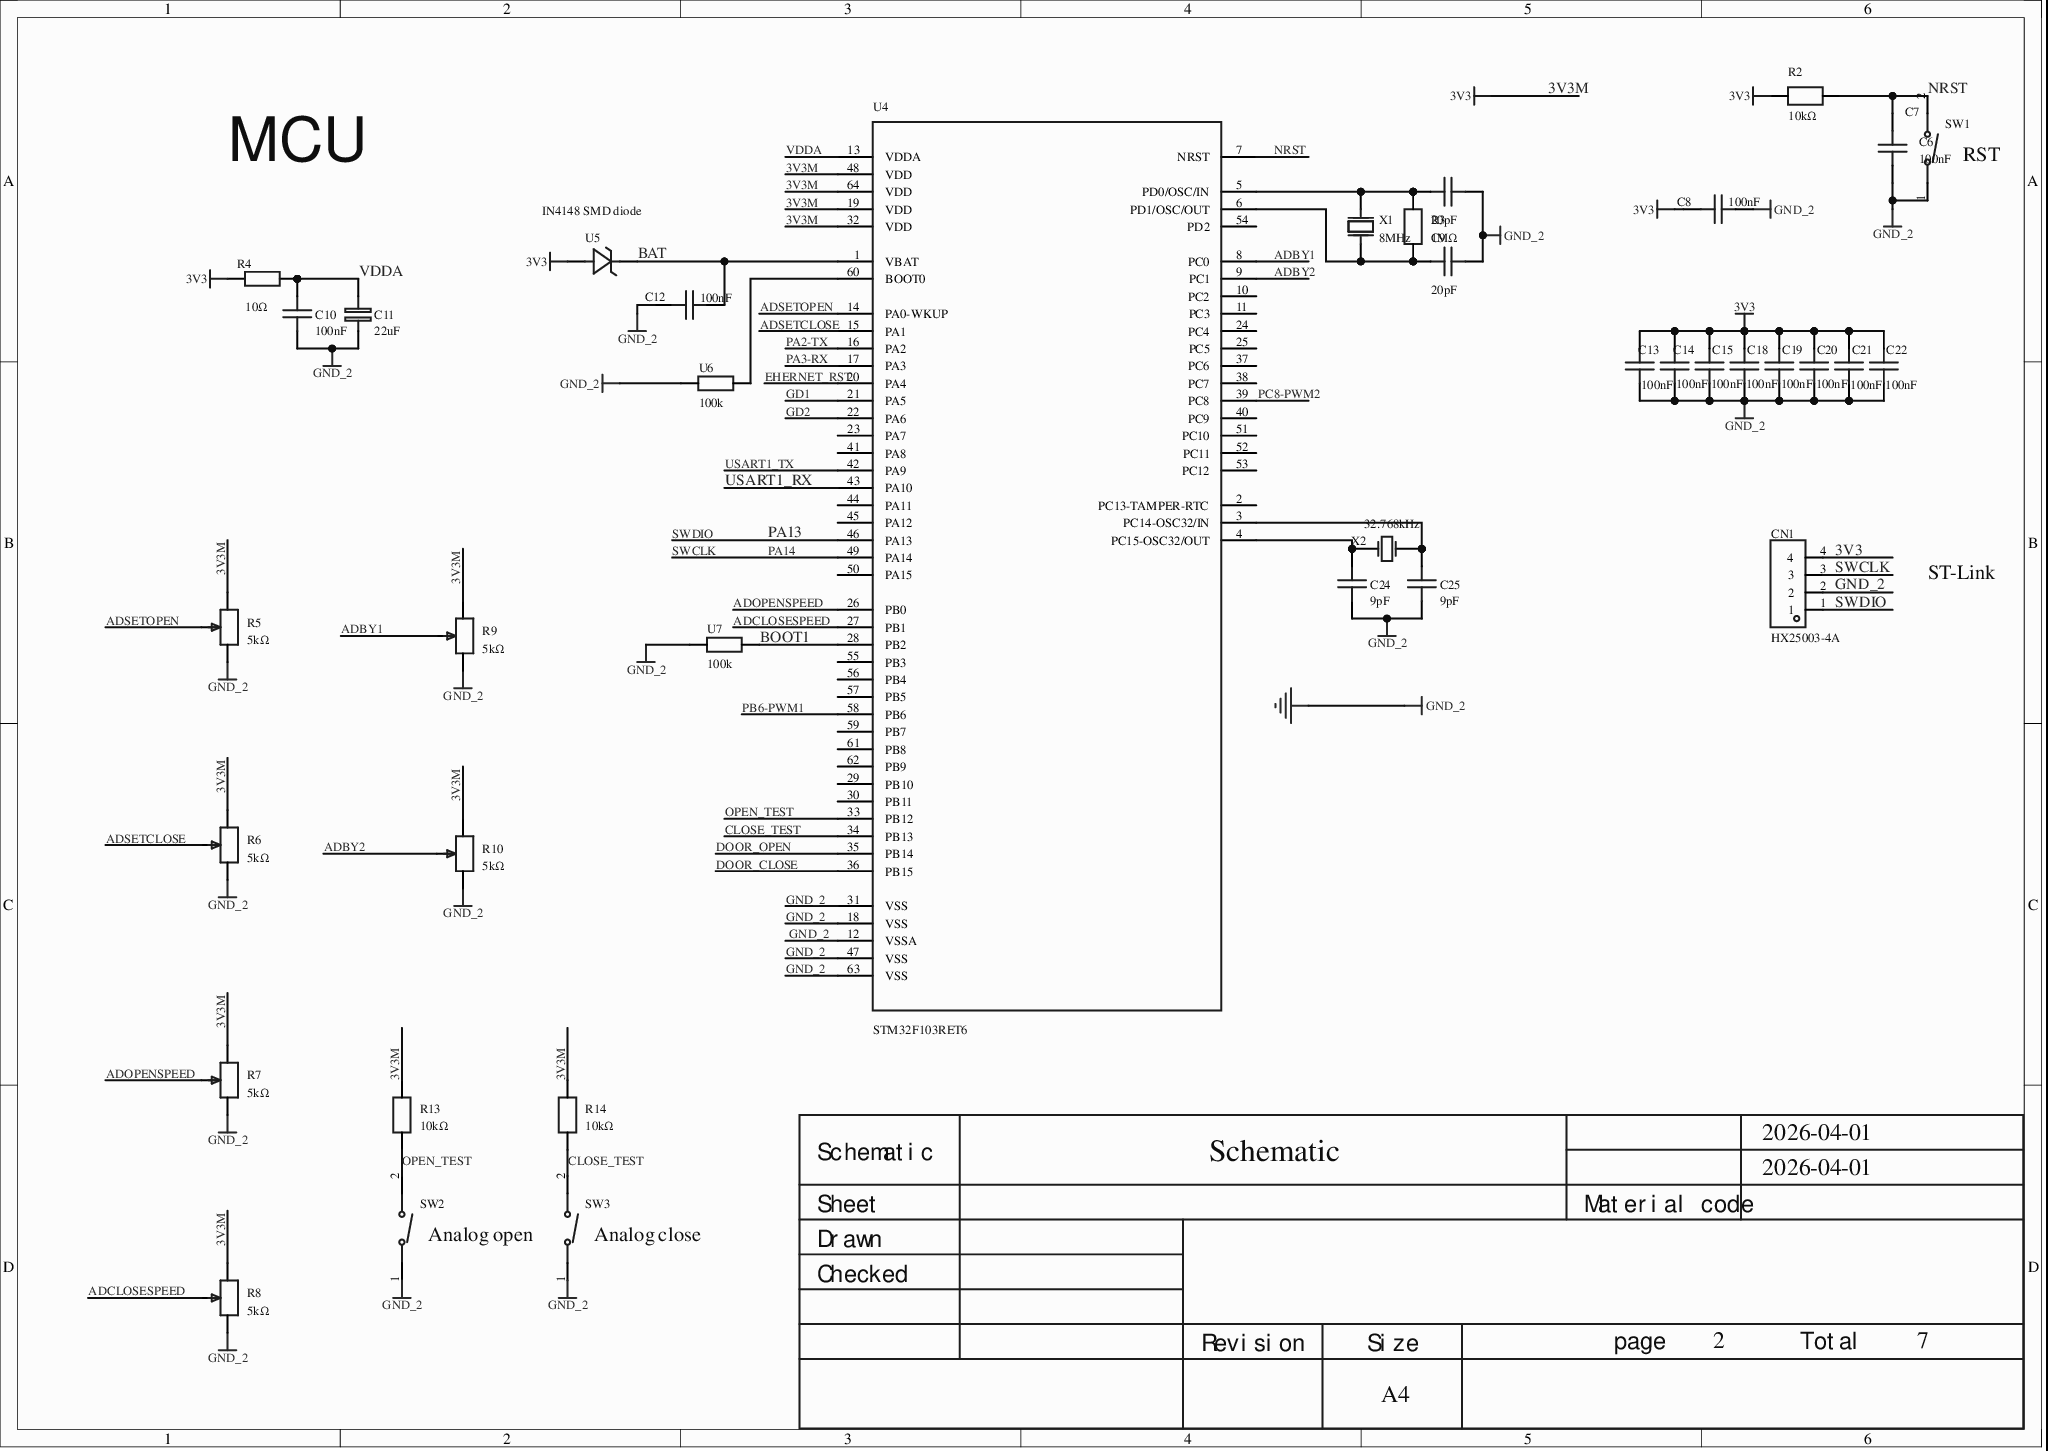
[diagram p0: MISC49876-3.schdoc]
# Altium project MISC49876-2.PrjPcb (part 1 of 2)
3 sheets, 90 parts. Net scope: global (net labels, ports and power ports of the same name join across sheets).
Board file: MISC49876.pcbdoc
Sheets:
  MISC49876-3.schdoc
  MISC49876-5.schdoc
  MISC49876-4.schdoc

## Sheet MISC49876-3.schdoc
size 297 x 210 mm; Version: V1.0; @Project Name: MISC49876; @Page Count: 7; @Update Date: 2026-04-01; @Create Date: 2026-04-01; @Schematic Name: MISC49876; @Page No: 2; @Board Name: MISC49876; @Create Time: 08:05:42; @Update Time: 16:05:42

### Parts
C6  100nF  [C0603]
C7  20pF  [C0603]
C8  100nF  [C0603]
C9  20pF  [C0603]
C10  100nF  [C0603]
C11  22uF  [C0603]
C12  100nF  [C0603]
C13  100nF  [C0603]
C14  100nF  [C0603]
C15  100nF  [C0603]
C18  100nF  [C0603]
C19  100nF  [C0603]
C20  100nF  [C0603]
C21  100nF  [C0603]
C22  100nF  [C0603]
C24  9pF  [C0402]
C25  9pF  [C0402]
CN1  HX25003-4A  [CONN-TH_4P-P2.50_HX25003-4A]
R2  10kΩ  [R0603]
R3  1MΩ  [R0603]
R4  10Ω  [R0603]
R5  5kΩ  [RES-ADJ-TH_3296W-1-203]
R6  5kΩ  [RES-ADJ-TH_3296W-1-203]
R7  5kΩ  [RES-ADJ-TH_3296W-1-203]
R8  5kΩ  [RES-ADJ-TH_3296W-1-203]
R9  5kΩ  [RES-ADJ-TH_3296W-1-203]
R10  5kΩ  [RES-ADJ-TH_3296W-1-203]
R13  10kΩ  [R0603]
R14  10kΩ  [R0603]
SW1  TS-1101-C-W  [SW-SMD_L6.0-W3.3-LS8.0]  (value not drawn)
SW2  TS-1101-C-W  [SW-SMD_L6.0-W3.3-LS8.0]  (value not drawn)
SW3  TS-1101-C-W  [SW-SMD_L6.0-W3.3-LS8.0]  (value not drawn)
U4  STM32F103RET6  [LQFP-64_L10.0-W10.0-P0.50-LS12.0-BL]
U5  IN4148 SMD diode  [SOD-123_L2.7-W1.7-LS3.8-RD]
U6  100k  [R0603]
U7  100k  [R0603]
X1  8MHz  [CRYSTAL-SMD_L11.5-W4.8-LS12.7]
X2  32.768kHz  [OSC-SMD_L3.2-W1.5]

### Nets
3V3: C8.1 C13.2 C14.2 C15.2 C18.2 C19.2 C20.2 C21.2 C22.2 CN1.4 R2.1 R4.1 R5.3 R6.3 R7.3 R8.3 R9.3 R10.3 R13.1 R14.1 U4.19(VDD) U4.32(VDD) U4.48(VDD) U4.64(VDD) U5.2(A)  [also labelled 3V3M]
GND_2: C6.2 C7.1 C8.2 C9.1 C10.1 C11.1 C12.1 C13.1 C14.1 C15.1 C18.1 C19.1 C20.1 C21.1 C22.1 C24.1 C25.1 CN1.2 R5.1 R6.1 R7.1 R8.1 R9.1 R10.1 SW1.1(A) SW2.1(A) SW3.1(A) U4.12(VSSA) U4.18(VSS) U4.31(VSS) U4.47(VSS) U4.63(VSS) U6.2 U7.1  [also labelled GND]
ADBY1: R9.2 U4.8(PC0)
ADBY2: R10.2 U4.9(PC1)
ADCLOSESPEED: R8.2 U4.27(PB1)
ADOPENSPEED: R7.2 U4.26(PB0)
ADSETCLOSE: R6.2 U4.15(PA1)
ADSETOPEN: R5.2 U4.14(PA0-WKUP)
BAT: C12.2 U4.1(VBAT) U5.1(K)
BOOT1: U4.28(PB2) U7.2
CLOSE_TEST: R14.2 SW3.2(B) U4.34(PB13)
DOOR_CLOSE: U4.36(PB15)
DOOR_OPEN: U4.35(PB14)
EHERNET_RST: U4.20(PA4)
GD1: U4.21(PA5)
GD2: U4.22(PA6)
NRST: C6.1 R2.2 SW1.2(B) U4.7(NRST)
OPEN_TEST: R13.2 SW2.2(B) U4.33(PB12)
PA2-TX: U4.16(PA2)
PA3-RX: U4.17(PA3)
PA13: CN1.1 U4.46(PA13)  [also labelled SWDIO]
PA14: CN1.3 U4.49(PA14)  [also labelled SWCLK]
PB6-PWM1: U4.58(PB6)
PC8-PWM2: U4.39(PC8)
USART1_RX: U4.43(PA10)
USART1_TX: U4.42(PA9)
VDDA: C10.2 C11.2 R4.2 U4.13(VDDA)
NetC7_2: C7.2 R3.1 U4.5(PD0/OSC/IN) X1.1(OSC1)
NetC9_2: C9.2 R3.2 U4.6(PD1/OSC/OUT) X1.2(OSC2)
NetC24_2: C24.2 U4.4(PC15-OSC32/OUT) X2.2(OSC2)
NetC25_2: C25.2 U4.3(PC14-OSC32/IN) X2.1(OSC1)
NetU4_60: U4.60(BOOT0) U6.1

Not connected (* = marked no-connect by the designer): U4 2(PC13-TAMPER-RTC) 10(PC2) 11(PC3) 23(PA7) 24(PC4) 25(PC5) 29(PB10) 30(PB11) 37(PC6) 38(PC7) 40(PC9) 41(PA8) 44(PA11) 45(PA12) 50(PA15) 51(PC10) 52(PC11) 53(PC12) 54(PD2) 55(PB3) 56(PB4) 57(PB5) 59(PB7) 61(PB8) 62(PB9)

### Notes on the sheet
- MCU
- (near SW1) RST
- ST-Link
- Analog open
- (near SW3) Analog close
- 2026-04-01
- Schematic
- Sheet
- Material code
- Checked
- Drawn
- Revision
- Size
- A4
- page
- 2
- Total
- 7

### Library data of the parts
C6 C8 C12-C15 C18-C22 = CC0603KRX7R9BB104: Capacitance: 100nF; tolerance: ±10%; rated voltage: 50V; dielectric (temp. coefficient): X7R;; Manufacturer: YAGEO(国巨); Symbol: 0.1u; Convert to PCB: yes; ModelId: ac125912035d415993ca9572d50418b1; ModelName: C0603_L1.6-W0.8-H0.8; ModelTransform: 62.992,31.496,0,0,0,0,0,0,0; Origin Footprint: C0603; Device: CC0603KRX7R9BB104; Supplier Part: C14663; Supplier: LCSC; Manufacturer Part: CC0603KRX7R9BB104; Add into BOM: yes; JLCPCB Part Class: Basic Part; LCSC Part Name: 100nF ±10% 50V; Supplier Footprint: 0603; Datasheet: https://atta.szlcsc.com/upload/public/pdf/source/20180910/C282072_33301C7F631E79921B82A8DAC6BCC5B3.pdf; FootprintName: C0603; Value: 100nF; Tolerance: ±10%; Voltage Rated: 50V; Temperature Coefficient: X7R
C7 C9 = CC0603JRNPO9BN200: Capacitance: 20pF; tolerance: ±5%; rated voltage: 50V; dielectric (temp. coefficient): NP0;; Manufacturer: YAGEO(国巨); Convert to PCB: yes; ModelId: ac125912035d415993ca9572d50418b1; ModelName: C0603_L1.6-W0.8-H0.8; ModelTransform: 62.992,31.496,0,0,0,0,0,0,0; Origin Footprint: C0603; Device: CC0603JRNPO9BN200; Symbol: 20pf; Supplier Part: C105621; Supplier: LCSC; Manufacturer Part: CC0603JRNPO9BN200; Add into BOM: yes; LCSC Part Name: 20pF ±5% 50V; Supplier Footprint: 0603; JLCPCB Part Class: Extended Part; Datasheet: https://atta.szlcsc.com/upload/public/pdf/source/20170505/1493957838062.pdf; FootprintName: C0603; Value: 20pF; Tolerance: ±5%; Voltage Rated: 50V; Temperature Coefficient: NP0
C10 = CC0603KRX7R9BB104: Capacitance: 100nF; tolerance: ±10%; rated voltage: 50V; dielectric (temp. coefficient): X7R;; Manufacturer: YAGEO(国巨); Symbol: 0.1u; Convert to PCB: yes; 3D Model: ac125912035d415993ca9572d50418b1; 3D Model Transform: 62.992,31.496,0,0,0,0,0,0,0; ModelName: C0603_L1.6-W0.8-H0.8; Origin Footprint: C0603; Device: CC0603KRX7R9BB104; Supplier Part: C14663; Supplier: LCSC; Manufacturer Part: CC0603KRX7R9BB104; Add into BOM: yes; JLCPCB Part Class: Basic Part; LCSC Part Name: 100nF ±10% 50V; Supplier Footprint: 0603; Datasheet: https://atta.szlcsc.com/upload/public/pdf/source/20180910/C282072_33301C7F631E79921B82A8DAC6BCC5B3.pdf; Value: 100nF; Tolerance: ±10%; Voltage Rated: 50V; Temperature Coefficient: X7R; FootprintName: C0603
C11 = CL10A226MQ8NRNC: Capacitance: 22uF; tolerance: ±20%; rated voltage: 6.3V; dielectric (temp. coefficient): X5R;; Manufacturer: SAMSUNG(三星); Origin Footprint: C0805; Convert to PCB: yes; 3D Model: ac125912035d415993ca9572d50418b1; 3D Model Transform: 62.992,31.496,0,0,0,0,0,0,0; ModelName: C0603_L1.6-W0.8-H0.8; Device: CL10A226MQ8NRNC; Symbol: 22uf; Supplier Part: C59461; Supplier: LCSC; Manufacturer Part: CL10A226MQ8NRNC; Add into BOM: yes; LCSC Part Name: 22uF ±20% 6.3V; Supplier Footprint: 0603; JLCPCB Part Class: Basic Part; Datasheet: https://atta.szlcsc.com/upload/public/pdf/source/20160218/1457707763339.pdf; Value: 22uF; Tolerance: ±20%; Voltage Rated: 6.3V; Temperature Coefficient: X5R; FootprintName: C0603
C24 C25 = 0402CG9R0C500NT: Capacitance: 9pF; rated voltage: 50V; dielectric (temp. coefficient): C0G;; Manufacturer: FH(风华); Origin Footprint: C0603; Symbol: 10pf; Convert to PCB: yes; Tolerance: ±5%; ModelId: 36a51122f27c49738f86b3bfa98863e0; ModelName: C0402_L1.0-W0.5-H0.5; ModelTransform: 39.37,19.685,0,0,0,0,0,0,0; Device: 0402CG9R0C500NT; Supplier Part: C1580; Supplier: LCSC; Manufacturer Part: 0402CG9R0C500NT; Add into BOM: yes; LCSC Part Name: 9pF 50V ±0.25pF; Supplier Footprint: 0402; JLCPCB Part Class: Extended Part; Datasheet: https://atta.szlcsc.com/upload/public/pdf/source/20200305/C486355_26A10D38EF8C2A5C37091D0039909270.pdf; FootprintName: C0402; Value: 9pF; Voltage Rated: 50V; Temperature Coefficient: C0G
CN1 = HX25003-4A: Pin structure: 1x4P; pitch: 2.5mm; gender: male; mounting: through-hole; row spacing: -; rows: 1; pins per row: 4; reference series: XH; rated current: -; operating temperature range: -;; Manufacturer: HX(红星); AddInBom: yes; ModelId: 7e25758d1952479b9526ef110128900c; ModelName: CONN-TH_XH2.50-LI-4P; ModelTransform: 492.125,224.409,0,0,0,0,0,-17.717,-118.11; Number of PINs Per Row: 4; Symbol: HX25003-4A; Device: HX25003-4A; Supplier: LCSC; Supplier Part: C442301; Manufacturer Part: HX25003-4A; JLCPCB Part Class: Extended library; LCSC Part Name: 1x4P 间距:2.5mm 直插 系列:XH 母座; Supplier Footprint: 插件,P=2.5mm; Datasheet: https://atta.szlcsc.com/upload/public/pdf/source/20191028/C442312_1520F9194999EF6509032948661325F7.pdf; ConvertToPcb: yes; FootprintName: CONN-TH_4P-P2.50_HX25003-4A; Pins Structure: 1x4P; Pitch: 2.5mm; Gender: Male; Mounting Style: Through-hole; Row Spacing: -; Number of Rows: 1; Reference Series: XH; Current Rating (Max): -; Operating Temperature Range: -
R2 = 0603WAF1002T5E: Resistance: 10kΩ; tolerance: ±1%; power: 100mW; temp. coefficient: ±100ppm/℃; resistor type: thick film resistor;; Manufacturer: UNI-ROYAL(厚声); Symbol: 10k; Convert to PCB: yes; ModelId: fc143cca1e79419f9cd78b61e9279f08; ModelTransform: 31.8897,63.7794,0,90,0,0,0,0,0; Overload Voltage (Max): 75V; Origin Footprint: R0603; Device: 0603WAF1002T5E; Supplier Part: C25804; Supplier: LCSC; Manufacturer Part: 0603WAF1002T5E; Add into BOM: yes; LCSC Part Name: 10kΩ ±1% 100mW 厚膜电阻; Supplier Footprint: 0603; JLCPCB Part Class: Basic Part; Datasheet: https://atta.szlcsc.com/upload/public/pdf/source/20200306/C422600_1E6D84923E4A46A82E41ADD87F860B5C.pdf; FootprintName: R0603; ModelName: R0603; Value: 10kΩ; Tolerance: ±1%; Power(Watts): 100mW; Temperature Coefficient: ±100ppm/℃; Type: Thick film resistor; Operating Temperature Range: -55℃~+155℃
R3 = 0603WAF1004T5E: Resistance: 1MΩ; tolerance: ±1%; power: 100mW; temp. coefficient: ±100ppm/℃; resistor type: thick film resistor;; Manufacturer: UNI-ROYAL(厚声); Symbol: 1m; Convert to PCB: yes; ModelId: fc143cca1e79419f9cd78b61e9279f08; ModelTransform: 31.8897,63.7794,0,90,0,0,0,0,0; Overload Voltage (Max): 75V; Origin Footprint: R0603; Device: 0603WAF1004T5E; Supplier Part: C22935; Supplier: LCSC; Manufacturer Part: 0603WAF1004T5E; Add into BOM: yes; LCSC Part Name: 1MΩ ±1% 100mW 厚膜电阻; Supplier Footprint: 0603; JLCPCB Part Class: Basic Part; Datasheet: https://atta.szlcsc.com/upload/public/pdf/source/20200306/C422600_1E6D84923E4A46A82E41ADD87F860B5C.pdf; FootprintName: R0603; ModelName: R0603; Value: 1MΩ; Tolerance: ±1%; Power(Watts): 100mW; Temperature Coefficient: ±100ppm/℃; Type: Thick film resistor; Operating Temperature Range: -55℃~+155℃
R4 = 0603WAF100JT5E: Resistance: 10Ω; tolerance: ±1%; power: 100mW; temp. coefficient: ±400ppm/℃; resistor type: thick film resistor;; Manufacturer: UNI-ROYAL(厚声); 3D Model: fc143cca1e79419f9cd78b61e9279f08; 3D Model Transform: 31.8897,63.7794,0,90,0,0,0,0,0; Overload Voltage (Max): 75V; AddInBom: yes; Symbol: 0603WAF100JT5E; Device: 0603WAF100JT5E; LCSC Part Name: 10Ω ±1% 100mW 厚膜电阻; Supplier Footprint: 0603; Datasheet: https://atta.szlcsc.com/upload/public/pdf/source/20200306/C422600_1E6D84923E4A46A82E41ADD87F860B5C.pdf; Tolerance: ±1%; Power(Watts): 100mW; Temperature Coefficient: ±400ppm/℃; Type: Thick film resistor; Operating Temperature Range: -55℃~+155℃; Supplier: LCSC; Manufacturer Part: 0603WAF100JT5E; Supplier Part: C22859; Value: 10Ω; JLCPCB Part Class: Basic library; ConvertToPcb: yes; FootprintName: R0603; ModelName: R0603
R5-R10 = 3296W-1-502_C48997929: Resistance: 5kΩ; tolerance: ±10%; power: 500mW; temp. coefficient: ±250ppm/℃;; Manufacturer: JIERR(捷而瑞); AddInBom: yes; ModelId: 308f73de4c8d41cbbdbfc058a8bb80b10819f05c4eef4c71ace90d822a990e87; ModelName: RES-ADJ-TH_3296W-L; ModelTransform: 374.015,190.9445,0,0,0,0,-0.001,-0.983,-196.85; Number of Turns: 28; Symbol: 3296W-1-502_C48997929; Device: 3296W-1-502_C48997929; LCSC Part Name: 玻璃釉预调电位器; SupplierPart: C48997929; ManufacturerPart: 3296W-1-502; Supplier Footprint: 插件-3P,9.5x4.9mm; JLCPCB Part Class: Extended Part; Datasheet: https://item.szlcsc.com/datasheet/3296W-1-502/51342065.html; Supplier: LCSC; ConvertToPcb: yes; FootprintName: RES-ADJ-TH_3296W-1-203; Value: 5kΩ; Tolerance: ±10%; Power(Watts): 500mW; Temperature Coefficient: ±250ppm/℃
R13 R14 = 0603WAF1002T5E: Resistance: 10kΩ; tolerance: ±1%; power: 100mW; temp. coefficient: ±100ppm/℃; resistor type: thick film resistor;; Manufacturer: UNI-ROYAL(厚声); Symbol: 10k; Add into BOM: yes; 3D Model: fc143cca1e79419f9cd78b61e9279f08; 3D Model Transform: 31.8897,63.7794,0,90,0,0,0,0,0; Overload Voltage (Max): 75V; Device: 0603WAF1002T5E; Convert to PCB: yes; Origin Footprint: R0603; Supplier Part: C25804; Supplier: LCSC; Manufacturer Part: 0603WAF1002T5E; LCSC Part Name: 10kΩ ±1% 100mW 厚膜电阻; Supplier Footprint: 0603; JLCPCB Part Class: Basic Part; Datasheet: https://atta.szlcsc.com/upload/public/pdf/source/20200306/C422600_1E6D84923E4A46A82E41ADD87F860B5C.pdf; Value: 10kΩ; Tolerance: ±1%; Power(Watts): 100mW; Temperature Coefficient: ±100ppm/℃; Type: Thick film resistor; Operating Temperature Range: -55℃~+155℃; FootprintName: R0603; ModelName: R0603
SW1 = TS-1101-C-W: 电路结构:单刀单掷;带支架:否;触点电流:50mA;额定电压(AC):-;额定电压(DC):12V;额定功率:-;安装方式:立贴;绝缘电阻:-;带灯:无;作用力:260gf;机械寿命:5万次;; Manufacturer: XKB Connectivity(中国星坤); Origin Footprint: SW-SMD_L6.0-W3.5-LS8.0-EH; Symbol: 1ts002c-2600-5001; Convert to PCB: yes; ModelId: b2f4ea9f0afc4b0786d53dba66ceb9e4; ModelName: SW-SMD_L6.0-W3.3-H5-LS8.0; ModelTransform: 314.96,129.921,0,0,0,0,0,0,0; Circuit: SPST; Actuator Style: Rectangular button; Switch Length: 6mm; Switch Width: 3.6mm; Switch Height: 2.5mm; Strike Gundam: No; Contact Current: 50mA; Voltage Rating (DC): 12V; Actuator/Cap Color: White with light green; With Lamp: None; Operating Force: 260gf; Mechanical Life: 5万次; Device: TS-1101-C-W; Supplier: LCSC; Supplier Part: C318938; Manufacturer Part: TS-1101-C-W; Add into BOM: yes; LCSC Part Name: 6*3.6*2.5mm 立贴 轻触开关 白色带淡绿按键 卷装; Supplier Footprint: SMD; JLCPCB Part Class: Extended Part; Datasheet: https://atta.szlcsc.com/upload/public/pdf/source/20200227/C318938_C2E53B1EEDE37D980A33616AC086DE53.pdf; FootprintName: SW-SMD_L6.0-W3.3-LS8.0; Voltage Rating (AC): -; Power Rating: -; Mounting Style: Surface mount; Insulation Resistance: -; IP Rating: -; Pin Style: -; Operating Temperature: -30℃~+85℃
SW2 SW3 = TS-1101-C-W: 电路结构:单刀单掷;带支架:否;触点电流:50mA;额定电压(AC):-;额定电压(DC):12V;额定功率:-;安装方式:立贴;绝缘电阻:-;带灯:无;作用力:260gf;机械寿命:5万次;; Manufacturer: XKB Connectivity(中国星坤); Symbol: 1ts002c-2600-5001; Add into BOM: yes; Origin Footprint: SW-SMD_L6.0-W3.5-LS8.0-EH; 3D Model: b2f4ea9f0afc4b0786d53dba66ceb9e4; 3D Model Transform: 314.96,129.921,0,0,0,0,0,0,0; Circuit: SPST; Actuator Style: Rectangular button; Switch Length: 6mm; Switch Width: 3.6mm; Switch Height: 2.5mm; Strike Gundam: No; Contact Current: 50mA; Voltage Rating (DC): 12V; Actuator/Cap Color: White with light green; With Lamp: None; Operating Force: 260gf; Mechanical Life: 5万次; ModelName: SW-SMD_L6.0-W3.3-H5-LS8.0; Device: TS-1101-C-W; Convert to PCB: yes; Supplier: LCSC; Supplier Part: C318938; Manufacturer Part: TS-1101-C-W; LCSC Part Name: 6*3.6*2.5mm 立贴 轻触开关 白色带淡绿按键 卷装; Supplier Footprint: SMD; JLCPCB Part Class: Extended Part; Datasheet: https://atta.szlcsc.com/upload/public/pdf/source/20200227/C318938_C2E53B1EEDE37D980A33616AC086DE53.pdf; Voltage Rating (AC): -; Power Rating: -; Mounting Style: Surface mount; Insulation Resistance: -; IP Rating: -; Pin Style: -; Operating Temperature: -30℃~+85℃; FootprintName: SW-SMD_L6.0-W3.3-LS8.0
U4 = STM32F103RET6: CPU core: CM3; program memory: 512KB; total RAM: 64KB; GPIO ports: 51; operating voltage: 2V~3.6V; max CPU frequency: 72MHz; program memory type: FLASH;; Manufacturer: ST(意法半导体); AddInBom: yes; ModelId: cd9de06618c44fcf82654c43a457f83c; ModelName: LQFP-64_L10.0-W10.0-H1.4-LS12.0-P0.50; ModelTransform: 472.441,472.441,0,0,0,0,0,0,0; GPIO Ports Number: 51; ADC (Bit): 12bit; Peripheral/Function: DMA; on-chip temperature sensor; PWM; Symbol: STM32F103RET6; Device: STM32F103RET6; LCSC Part Name: STM32F103RET6; SupplierPart: C8322; ManufacturerPart: STM32F103RET6; Supplier Footprint: LQFP-64(10x10); JLCPCB Part Class: Extended library; Datasheet: https://atta.szlcsc.com/upload/public/pdf/source/20180327/C88435_0E51D69B5FFD7B1A3F36EB9FC047A4C2.pdf; Supplier: LCSC; ConvertToPcb: yes; FootprintName: LQFP-64_L10.0-W10.0-P0.50-LS12.0-BL; CPU Core: CM3; Program Storage Size: 512KB; RAM Size: 64KB; Operating Voltage Range: 2V~3.6V; CPU Maximum Speed: 72MHz; Program Memory Type: FLASH; Operating Temperature Range: -40℃~+85℃; DAC (Bit): 12bit; PWM (Bit): -; Universal Serial Bus: Yes; Internal Comparator: -; communication protocol: -; Watchdog: Yes; Real-Time Clock: -; Infrared Data Association: Yes; Low-Voltage Detect: Yes; CCP Capture/Compare: -; Secure Digital Input and Output: -; Direct Memory Access: Yes; Internal Oscillator: Yes
U5 = IN4148贴片二极管: AddInBom: yes; ModelId: b455d3bf1dad47d3a75f9a76b08071c6; ModelTransform: 145.669,64.961,0,0,0,0,0,0,0; JLCPCB Part Class: Extended Part; Device: IN4148 SMD diode; Symbol: IN4148 SMD diode; LCSC Part Name: IN4148贴片二极管; SupplierPart: C9900004332; ManufacturerPart: IN4148贴片二极管; Supplier Footprint: SOD123; Datasheet: https://example.com/datasheet; Supplier: LCSC; ConvertToPcb: yes; FootprintName: SOD-123_L2.7-W1.7-LS3.8-RD; ModelName: SOD-123_L2.7-W1.7-LS3.8-RD
U6 U7 = 100k: AddInBom: yes; ModelId: fc143cca1e79419f9cd78b61e9279f08; ModelTransform: 31.8897,63.7794,0,90,0,0,0,0,0; Device: 100k; Symbol: 100K; LCSC Part Name: 100k; SupplierPart: C9900012835; ManufacturerPart: 100k; Supplier Footprint: R0603; JLCPCB Part Class: Extended library; Supplier: LCSC; ConvertToPcb: yes; FootprintName: R0603; ModelName: R0603
X1 = X49SM8MSD2SC: Frequency: 8MHz; load capacitance: 20pF; frequency tolerance: ±20ppm;; Manufacturer: YXC(扬兴晶振); Origin Footprint: HC-49S_L11.4-W4.8; Convert to PCB: yes; ModelId: 6f569b91267b44029b8615eb5c810fba; ModelName: HC-49S_L11.4-W1.8-H3.0-LS12.7; ModelTransform: 499.999,188.976,0,180,0,0,0.002,-0.002,0; Crystal Type: 49SMD; Frequency Stability: ±30ppm; Device: X49SM8MSD2SC; Symbol: 8mhz; Supplier: LCSC; Supplier Part: C12674; Manufacturer Part: X49SM8MSD2SC; Add into BOM: yes; LCSC Part Name: 8MHz ±20ppm 20pF HC-49SMD; Supplier Footprint: HC-49S-SMD; JLCPCB Part Class: Basic Part; Datasheet: https://atta.szlcsc.com/upload/public/pdf/source/20210329/C106809_0E91E60850A780B284B63D653DC40EA4.pdf; FootprintName: CRYSTAL-SMD_L11.5-W4.8-LS12.7; Value: 8MHz; Load Capacitance: 20pF; Frequency Tolerance: ±20ppm; Operating Temperature: -20℃~+70℃
X2 = SC-32S32.768kHz20PPM12.5pF: Frequency: 32.768kHz; load capacitance: 12.5pF; frequency tolerance: ±20ppm;; Manufacturer: Seiko(精工); Origin Footprint: OSC-TH_BD2.0-P0.70-D0.3; Convert to PCB: yes; ModelId: 2dd241c0893b4675b8def6f6998a8251; ModelName: OSC-SMD_L3.2-W1.5-H0.8; ModelTransform: 125.984,59.055,0,0,0,0,0,-0.0005,0; Device: SC-32S32.768kHz20PPM12.5pF; Symbol: 32.768khz; Supplier: LCSC; Manufacturer Part: SC-32S32.768kHz20PPM12.5pF; Supplier Part: C97606; Add into BOM: yes; LCSC Part Name: 32.768kHz ±20ppm 12.5pF; Supplier Footprint: SMD3215-2P; JLCPCB Part Class: Extended Part; Datasheet: https://atta.szlcsc.com/upload/public/pdf/source/20170713/C97606_1499914220652816606.pdf; FootprintName: OSC-SMD_L3.2-W1.5; Crystal Type: -; Value: 32.768kHz; Load Capacitance: 12.5pF; Frequency Tolerance: ±20ppm; Operating Temperature: -

## Sheet MISC49876-5.schdoc
size 297 x 210 mm; Version: V1.0; @Project Name: MISC49876; @Page Count: 7; @Update Date: 2026-04-01; @Create Date: 2026-04-01; @Schematic Name: MISC49876; @Page No: 4; @Board Name: MISC49876; @Create Time: 08:05:42; @Update Time: 16:05:42
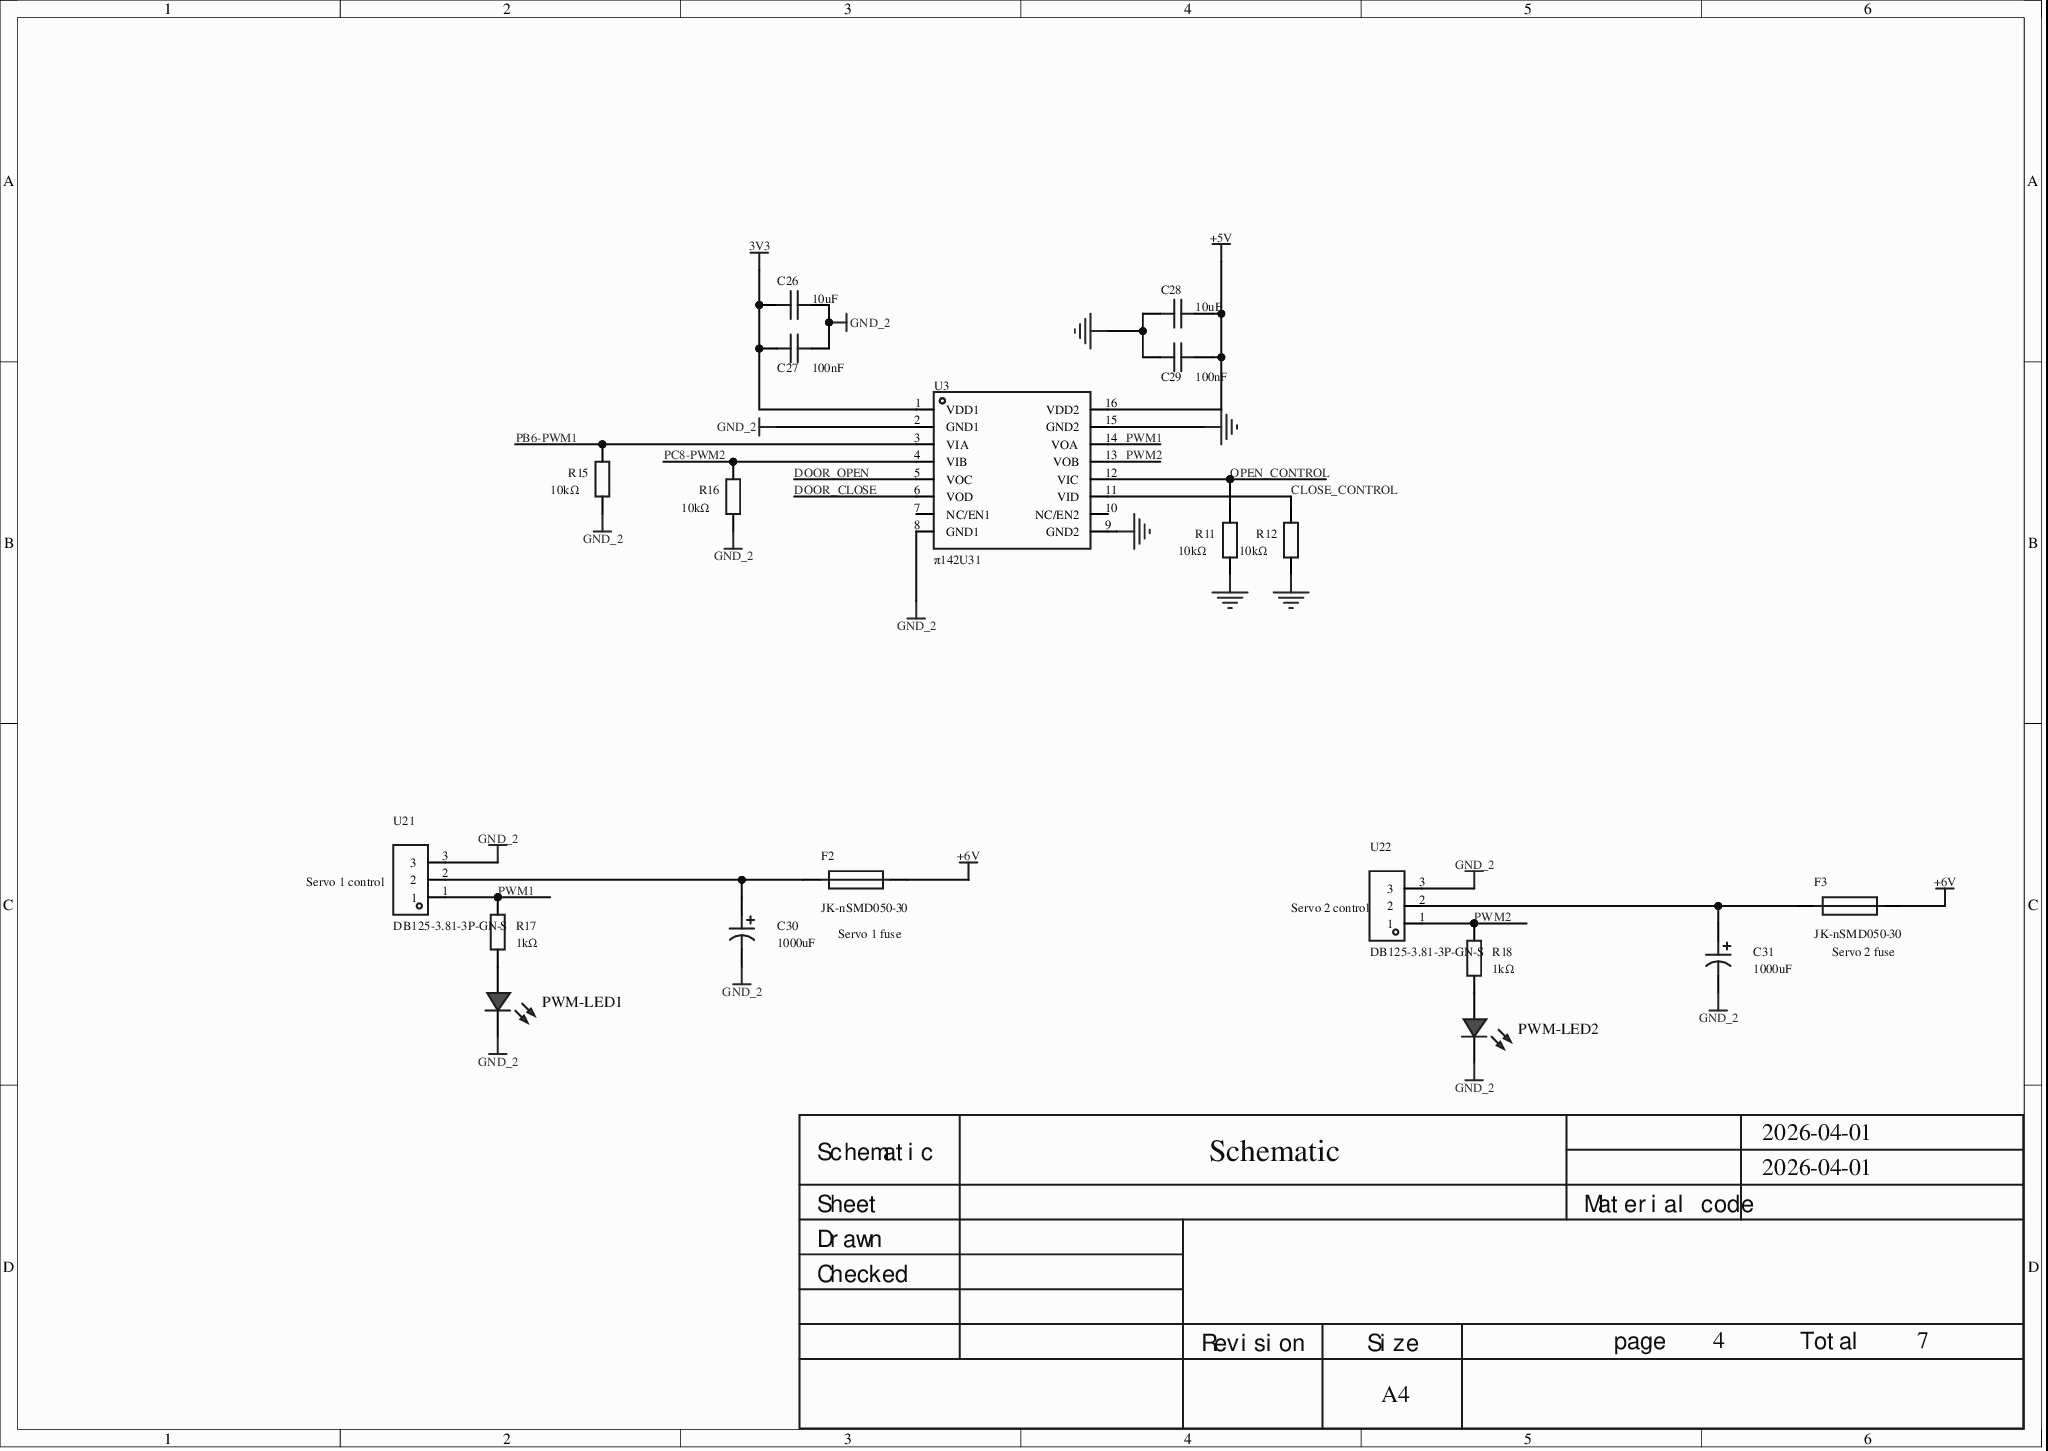
[diagram p1: MISC49876-5.schdoc]

### Parts
C26  10uF  [C0805]
C27  100nF  [C0603]
C28  10uF  [C0805]
C29  100nF  [C0603]
C30  1000uF  [CAP-TH_BD6.3-P2.50-D0.5-FD]
C31  1000uF  [CAP-TH_BD6.3-P2.50-D0.5-FD]
F2  JK-nSMD050-30  [F1206]
F3  JK-nSMD050-30  [F1206]
PWM-LED1  (no value)  [LED_0603]
PWM-LED2  (no value)  [LED_0603]
R11  10kΩ  [R0603]
R12  10kΩ  [R0603]
R15  10kΩ  [R0603]
R16  10kΩ  [R0603]
R17  1kΩ  [R0603]
R18  1kΩ  [R0603]
U3  π142U31  [SOIC-16_L9.9-W3.9-P1.27-LS6.0-BL]
U21  DB125-3.81-3P-GN-S  [CONN-TH_3P-P3.81_L7.4-W11.4]
U22  DB125-3.81-3P-GN-S  [CONN-TH_3P-P3.81_L7.4-W11.4]

### Nets
3V3: C26.1 C27.2 U3.1(VDD1)
+5V: C28.2 C29.1 U3.16(VDD2)
+6V: F2.2 F3.2
GND_2: C26.2 C27.1 C28.1 C29.2 C30.2 C31.2 PWM-LED1.1(C) PWM-LED2.1(C) R11.1 R12.1 R15.1 R16.1 U3.2(GND1) U3.8(GND1) U3.9(GND2) U3.15(GND2) U21.3 U22.3  [also labelled GND]